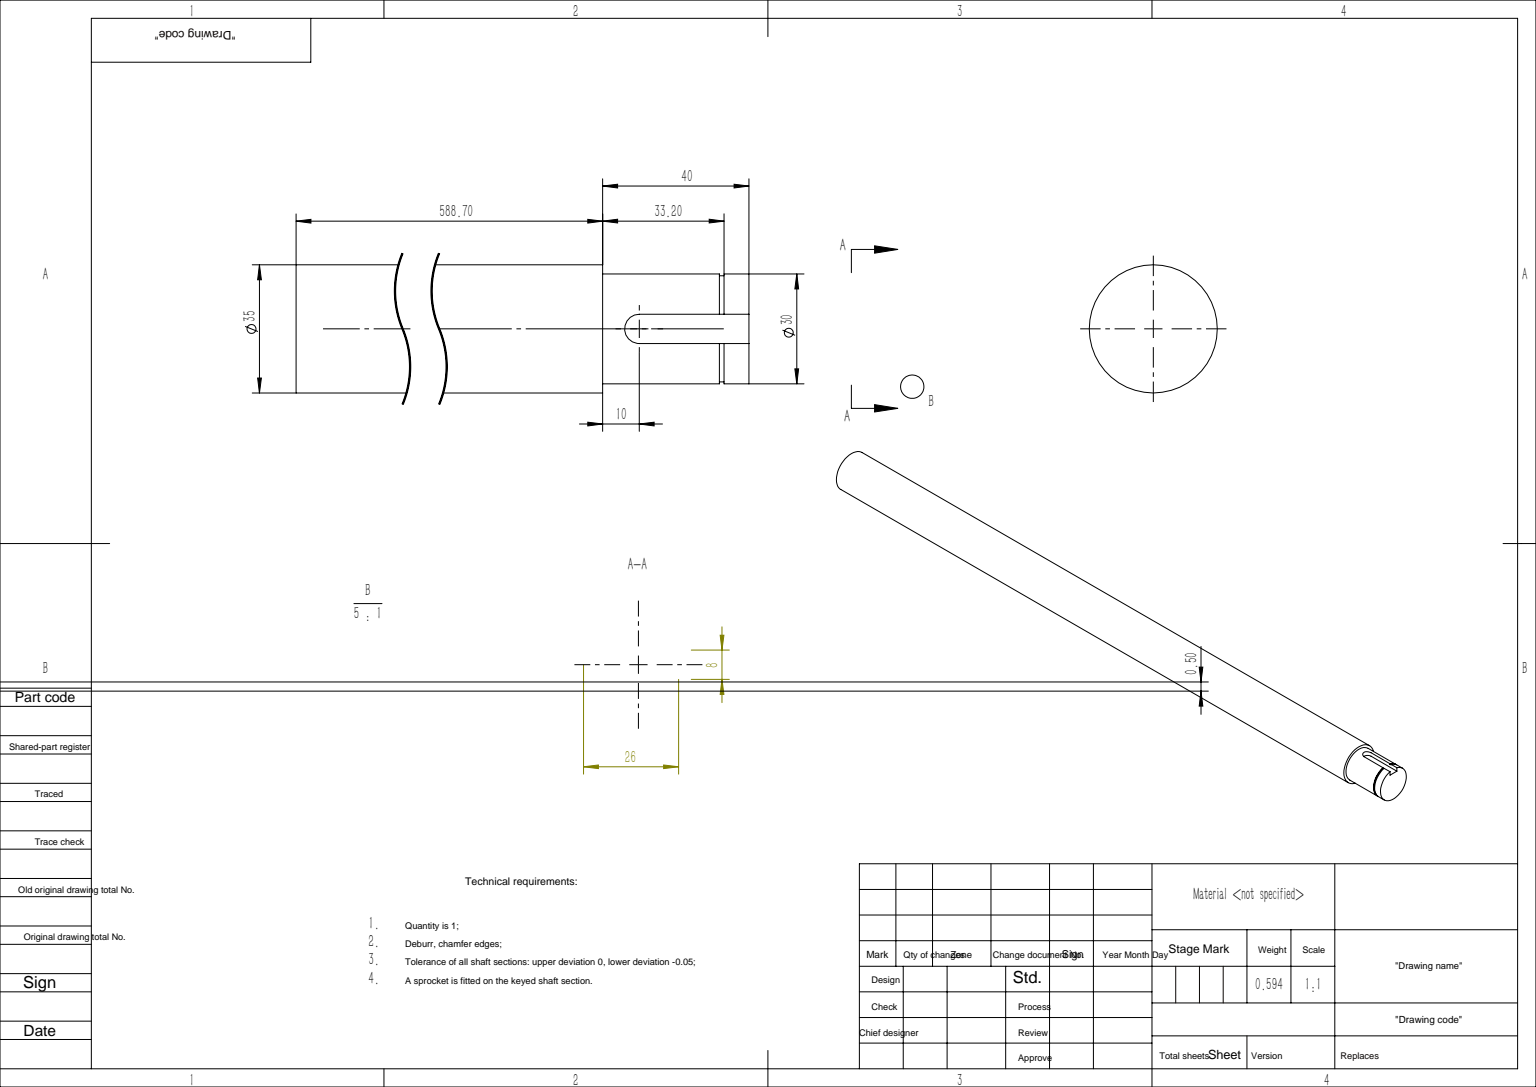
SolidWorks part; units mm, degrees
ref_plane "前视基准面" through (0, 0, 0) normal (0, 0, 1) x (1, 0, 0)
ref_plane "上视基准面" through (0, 0, 0) normal (0, 1, 0) x (1, 0, 0)
ref_plane "右视基准面" through (0, 0, 0) normal (1, 0, 0) x (0, 0, -1)
sketch "草图1" plane through (0, 0, 0) normal (1, 0, 0) x (0, 0, -1)
  circle A0 centre (0, 0) radius 17.5
  dimension "D1" = 35
extrude "凸台-拉伸1" add sketch "草图1" along normal blind 628.7
ref_plane "基准面1" through (544.5, -163.1345, -203.4942) normal (0, -0.365, -0.931) x (-1, 0, 0)
sketch "草图3" plane through (628.7, 0, 0) normal (1, 0, 0) x (0, 0, -1)
  circle A0 centre (0, 0) radius 17.5 construction
  circle A1 centre (0, 0) radius 17.5
  circle A2 centre (0, 0) radius 15
  dimension "D1" = 30
extrude "切除-拉伸1" cut sketch "草图3" against normal blind 40
ref_plane "基准面2" through (0, 15, 0) normal (0, 1, 0) x (1, 0, 0)
sketch "草图4" plane through (0, 15, 0) normal (0, 1, 0) x (1, 0, 0)
  line L0 (628.7, 0) -> (547.5705, 0) construction
  line L1 (628.7, -15) -> (628.7, 15) construction
  line L2 (598.7, 4) -> (628.7, 4)
  line L3 (598.7, -4) -> (628.7, -4)
  line L4 (628.7, 4) -> (628.7, -4)
  line L5 (588.7, -17.5) -> (588.7, 17.5) construction
  arc A0 (598.7, 4) -> (598.7, -4) centre (598.7, 0) ccw
  dimension "D2" = 4
  dimension "D1" = 10
extrude "切除-拉伸2" cut sketch "草图4" against normal blind 4
sketch "草图5" plane through (588.7, 0, 0) normal (1, 0, 0) x (0, 0, -1)
  circle A0 centre (0, 0) radius 15
  arc A1 (-4, 14.4568) -> (4, 14.4568) centre (0, 0) ccw construction
  circle A2 centre (0, 0) radius 14.5
  dimension "D1" = 0.5
extrude "切除-拉伸3" cut sketch "草图5" against normal blind 1.3 from offset 33.2
